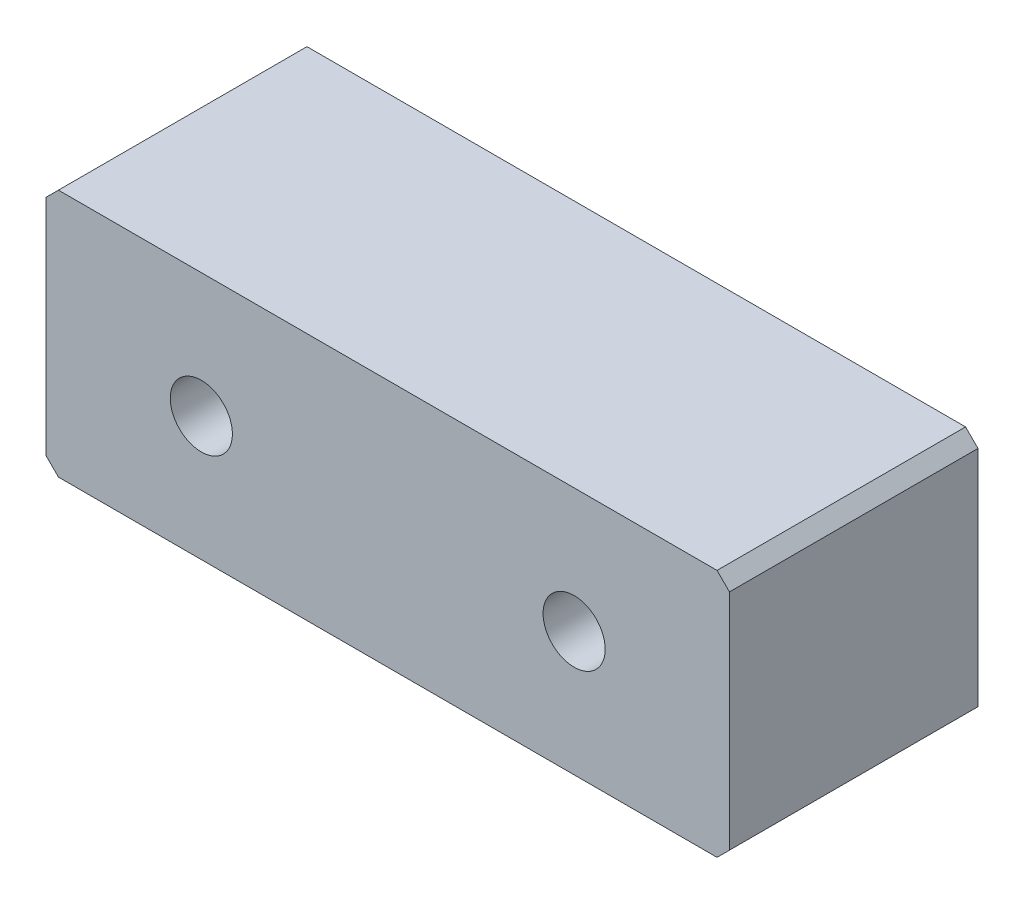
from build123d import *

# Parameters (mm, degrees)
SKETCH1_W           = 55
SKETCH1_H           = 20
BOSS_EXTRUDE1_DEPTH = 20
M6_TAPPED_HOLE1_D   = 5
CHAMFER1_SIZE       = 1


with BuildPart() as part:
    # Sketch1 → Boss-Extrude1 (new body)
    with BuildSketch(Plane.XY):
        with Locations((-52.336320298, 28.055555556)):
            Rectangle(SKETCH1_W, SKETCH1_H)
    extrude(amount=BOSS_EXTRUDE1_DEPTH)

    # M6 Tapped Hole1 (through all)
    with Locations(Plane.XY.offset(20)):
        with Locations((-67.336320298, 28.055555556), (-37.336320298, 28.055555556)):
            Hole(M6_TAPPED_HOLE1_D / 2)

    # Chamfer1
    chamfer1_edges = [part.edges().sort_by_distance(p)[0] for p in [
        (-79.836320298, 38.055555556, 10),
        (-24.836320298, 38.055555556, 10),
        (-24.836320298, 18.055555556, 10),
        (-79.836320298, 18.055555556, 10),
    ]]
    chamfer(chamfer1_edges, length=CHAMFER1_SIZE)


solid = part.part
